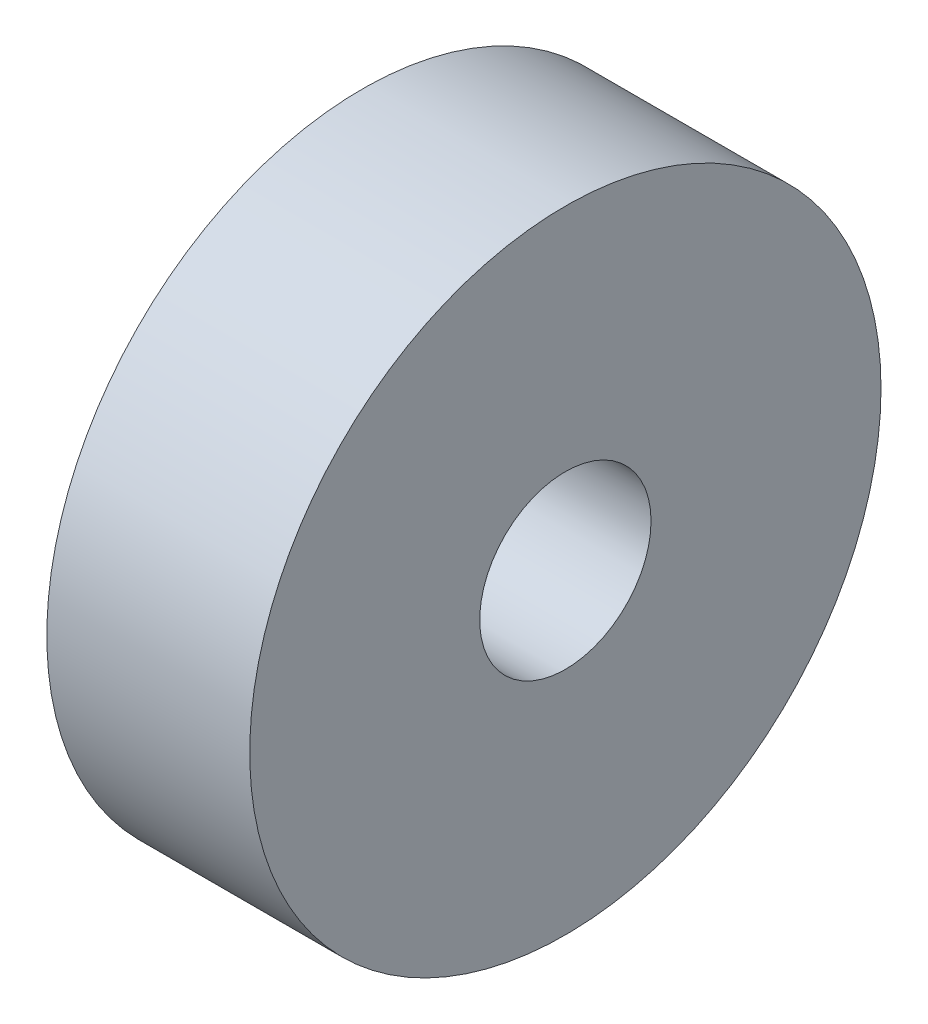
SolidWorks part; units mm, degrees
material "AISI 1045 钢，冷拔"
ref_plane "Front Plane" through (0, 0, 0) normal (0, 0, 1) x (1, 0, 0)
ref_plane "Top Plane" through (0, 0, 0) normal (0, 1, 0) x (1, 0, 0)
ref_plane "Right Plane" through (0, 0, 0) normal (1, 0, 0) x (0, 0, -1)
sketch "Sketch1" plane through (0, 0, 0) normal (0, 0, 1) x (1, 0, 0)
  line L0 (71.9012, 0) -> (0, 0) construction
  line L1 (0, 0) -> (0, 101.4822) construction
  line L3 (-45, 38) -> (45, 38)
  line L4 (-45, 38) -> (-45, 140)
  line L5 (-45, 140) -> (45, 140)
  line L6 (45, 38) -> (45, 140)
  line L7 (-45, 38) -> (45, 140) construction
  line L8 (-45, 140) -> (45, 38) construction
  point P3 (0, 89)
  dimension "D1" = 90
  dimension "D2" = 280
  dimension "D3" = 76
revolve "Revolve1" add sketch "Sketch1" angle 360 about L0
